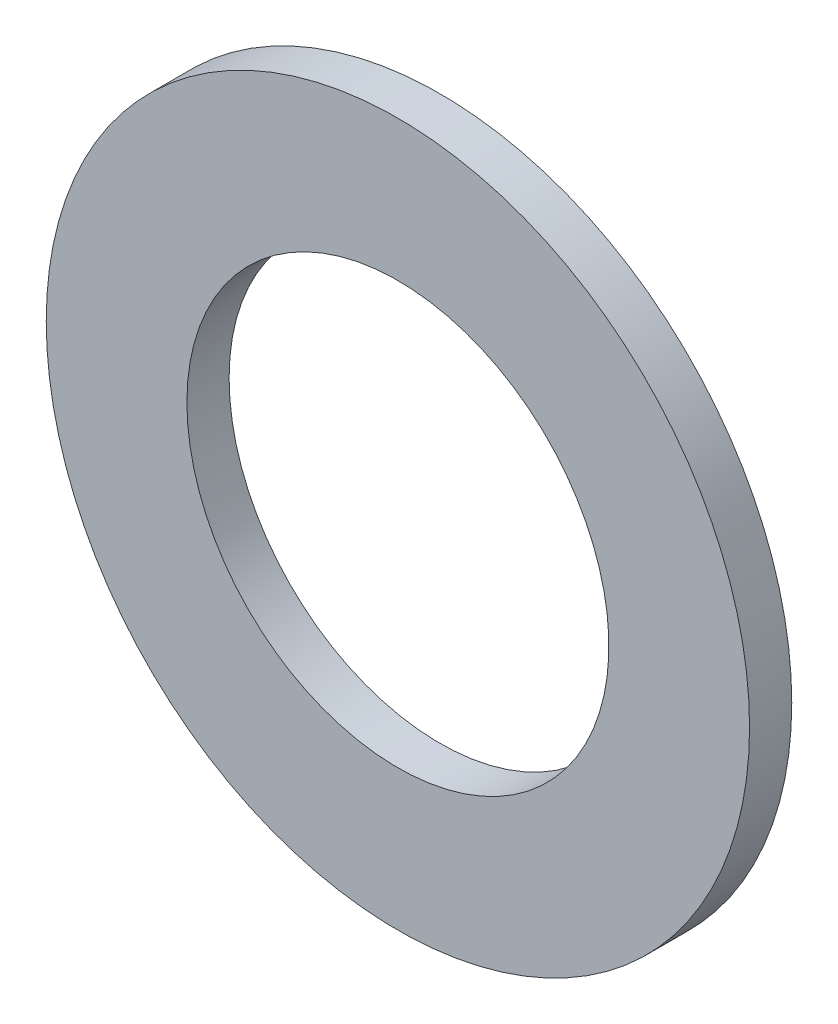
SolidWorks part; units mm, degrees
ref_plane "Front plane" through (0, 0, 0) normal (0, 0, 1) x (1, 0, 0)
ref_plane "Top plane" through (0, 0, 0) normal (0, 1, 0) x (1, 0, 0)
ref_plane "Right plane" through (0, 0, 0) normal (1, 0, 0) x (0, 0, -1)
sketch "Sketch 1" plane through (0, 0, 0) normal (0, 0, 1) x (1, 0, 0)
  circle A0 centre (0, 0) radius 2.5
  dimension "D1" = 5
extrude "Boss-Extrude 1" add sketch "Sketch 1" along normal blind 0.3
sketch "Sketch 2" plane through (0, 0, 0) normal (0, 0, -1) x (-1, 0, 0)
  circle A0 centre (0, 0) radius 1.5
  dimension "D1" = 3
extrude "Cut-Extrude 1" cut sketch "Sketch 2" against normal blind 0.3
